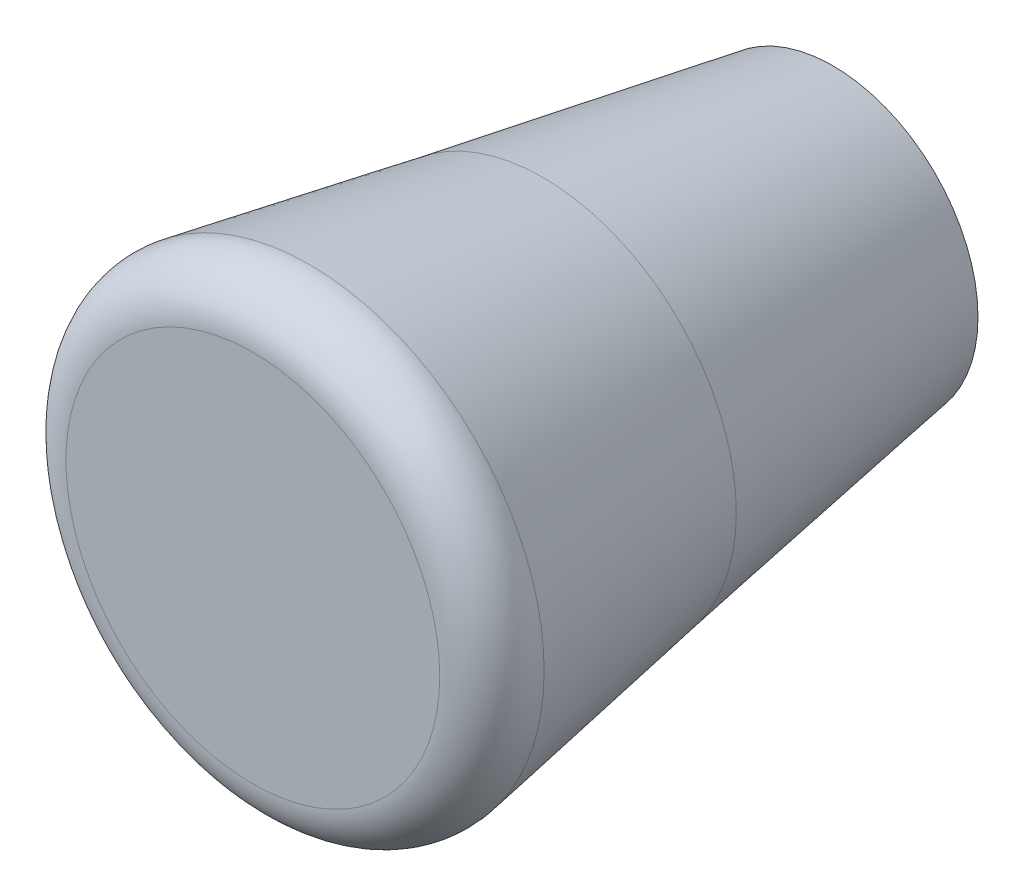
from build123d import *

# Parameters (mm, degrees)
SKETCH_1_3_R        = 20
BOSS_EXTRUDE1_DEPTH = 30
BOSS_EXTRUDE1_DRAFT = -10
SKETCH_1_3_2_R      = 20
SKETCH_1_3_2_R_2    = 15
BOSS_EXTRUDE2_DEPTH = 30
FILLET1_R           = 5


with BuildPart() as part:
    # Sketch 1_3 → Boss-Extrude1 (with draft: the straight prism first)
    with BuildSketch(Plane.XY):
        Circle(SKETCH_1_3_R)
    extrude(amount=BOSS_EXTRUDE1_DEPTH)
    # Boss-Extrude1: the draft: its side faces are tilted about the plane it starts from
    boss_extrude1_sides = [part.faces().sort_by_distance(p)[0] for p in [
        (-20, 0, 15),
    ]]
    draft(boss_extrude1_sides, Plane.XY, BOSS_EXTRUDE1_DRAFT)

    # Sketch 1_3 2 → Boss-Extrude2 (add)
    with BuildSketch(Plane.XY):
        Circle(SKETCH_1_3_2_R)
        Circle(SKETCH_1_3_2_R_2, mode=Mode.SUBTRACT)
    extrude(amount=-BOSS_EXTRUDE2_DEPTH)

    # Sketch2 → Cut-Revolve1 (revolve, cut)
    with BuildSketch(Plane(origin=(0, 0, 0), x_dir=(1, 0, 0), z_dir=(0, 1, 0))):
        Polygon((20, 0), (15, 30), (20, 30), align=None)
    revolve(axis=Axis((0, 0, 0), (0, 0, -1)), mode=Mode.SUBTRACT)

    # Fillet1
    fillet1_edges = [part.edges().sort_by_distance(p)[0] for p in [
        (-25.289809421, 0, 30),
    ]]
    fillet(fillet1_edges, radius=FILLET1_R)


solid = part.part
